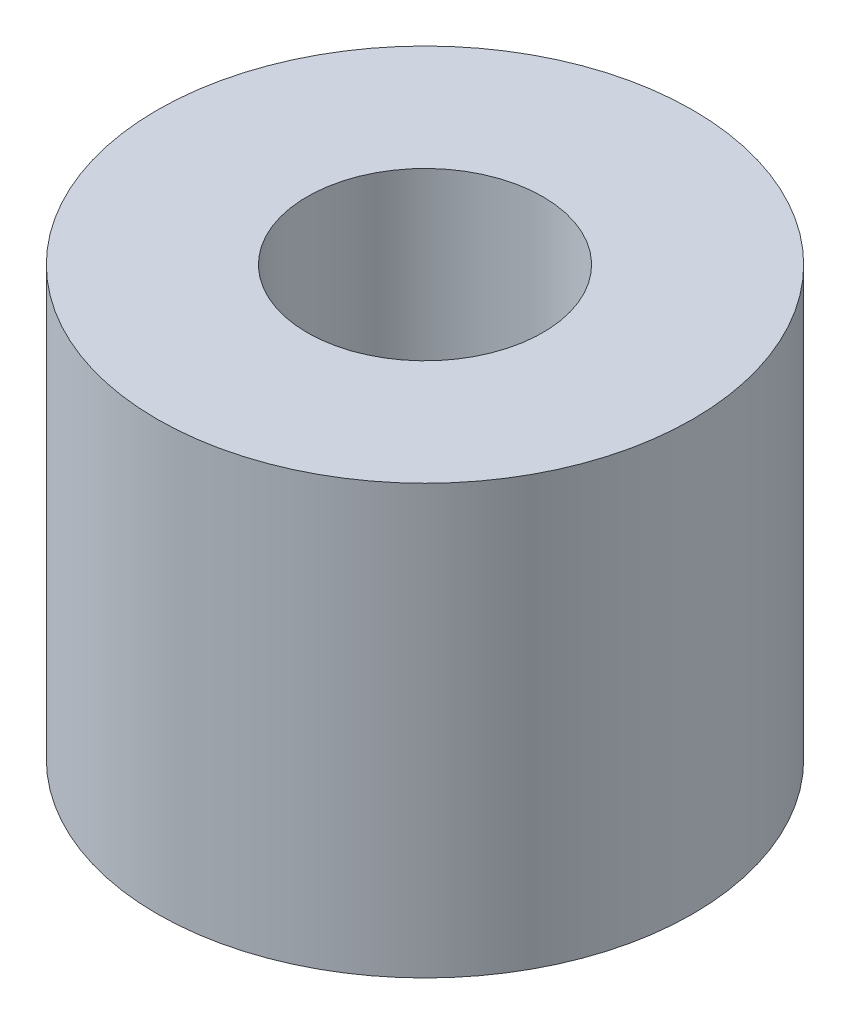
SolidWorks part; units mm, degrees
ref_plane "前视基准面" through (0, 0, 0) normal (0, 0, 1) x (1, 0, 0)
ref_plane "上视基准面" through (0, 0, 0) normal (0, 1, 0) x (1, 0, 0)
ref_plane "右视基准面" through (0, 0, 0) normal (1, 0, 0) x (0, 0, -1)
sketch "草图1" plane through (0, 0, 0) normal (0, 1, 0) x (1, 0, 0)
  circle A0 centre (0, 0) radius 12.5
  dimension "D1" = 25
extrude "凸台-拉伸1" add sketch "草图1" along normal blind 20
sketch "草图4" plane through (0, 20, 0) normal (0, 1, 0) x (1, 0, 0)
  point P0 (0, 0)
hole_wizard "M6 六角圆柱头螺钉的柱形沉头孔1" positions "草图4" profile "草图3" counterbore size "M6" standard "GB" end condition through all
sketch "草图3" plane through (0, 20, 0) normal (1, 0, 0) x (0, 0, 1)
  line L0 (0, 0) -> (0, 20)
  line L1 (0, 20) -> (3.3, 20)
  line L3 (3.3, 20) -> (3.3, 10.8)
  line L4 (3.3, 10.8) -> (5.5, 10.8)
  line L5 (5.5, 10.8) -> (5.5, 0)
  line L7 (5.5, 0) -> (0, 0)
  line L11 (0, -6.35) -> (0, 107.95) construction
  dimension "通孔孔直径" = 6.6
  dimension "通孔孔深度" = 20
  dimension "柱形沉头孔直径" = 11
  dimension "柱形沉头孔深度" = 10.8
